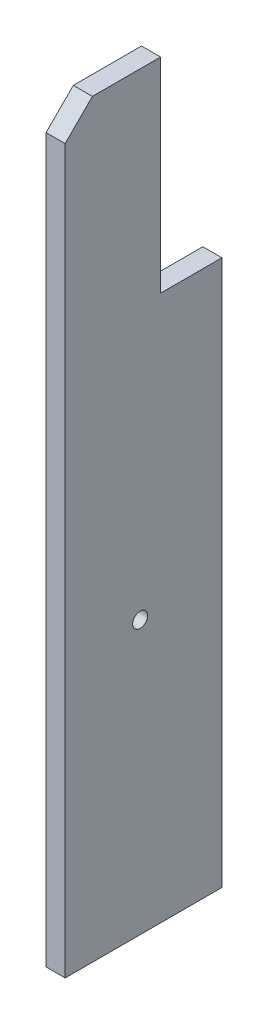
SolidWorks part; units mm, degrees
ref_plane "前视基准面" through (0, 0, 0) normal (0, 0, 1) x (1, 0, 0)
ref_plane "上视基准面" through (0, 0, 0) normal (0, 1, 0) x (1, 0, 0)
ref_plane "右视基准面" through (0, 0, 0) normal (1, 0, 0) x (0, 0, -1)
sketch "草图1" plane through (0, 0, 0) normal (1, 0, 0) x (0, 0, -1)
  line L0 (0, 0) -> (45, 0)
  line L1 (45, 0) -> (45, -400)
  line L2 (45, -400) -> (-70, -400)
  line L3 (-70, -400) -> (-70, 150)
  line L4 (-70, 150) -> (0, 150)
  line L5 (0, 150) -> (0, 0)
  dimension "D1" = 45
  dimension "D2" = 70
  dimension "D3" = 150
  dimension "D4" = 400
extrude "凸台-拉伸1" add sketch "草图1" along normal mid plane 14
sketch "草图2" plane through (7, 0, 0) normal (1, 0, 0) x (0, 0, -1)
  line L0 (-70, 150) -> (-70, -400) construction
  line L1 (-70, -400) -> (45, -400) construction
  line L2 (45, 0) -> (0, 0) construction
  line L3 (45, -400) -> (45, 0) construction
  circle A0 centre (20, -100) radius 5.5
  circle A1 centre (-45, -300) radius 5.5
  dimension "D1" = 11
  dimension "D2" = 11
  dimension "D3" = 25
  dimension "D4" = 100
  dimension "D5" = 100
  dimension "D6" = 25
extrude "切除-拉伸1" [suppressed] cut sketch "草图2" against normal up to next
sketch "草图3" plane through (7, 0, 0) normal (1, 0, 0) x (0, 0, -1)
  line L2 (-70, 150) -> (-70, -400) construction
  line L3 (-70, -400) -> (45, -400) construction
  circle A1 centre (-15, -200) radius 5.5
  dimension "D1" = 11
  dimension "D4" = 55
  dimension "D5" = 200
extrude "切除-拉伸2" cut sketch "草图3" against normal up to next
chamfer "倒角1" distance 20 angle 45 1 edges at (0, 150, 70)
